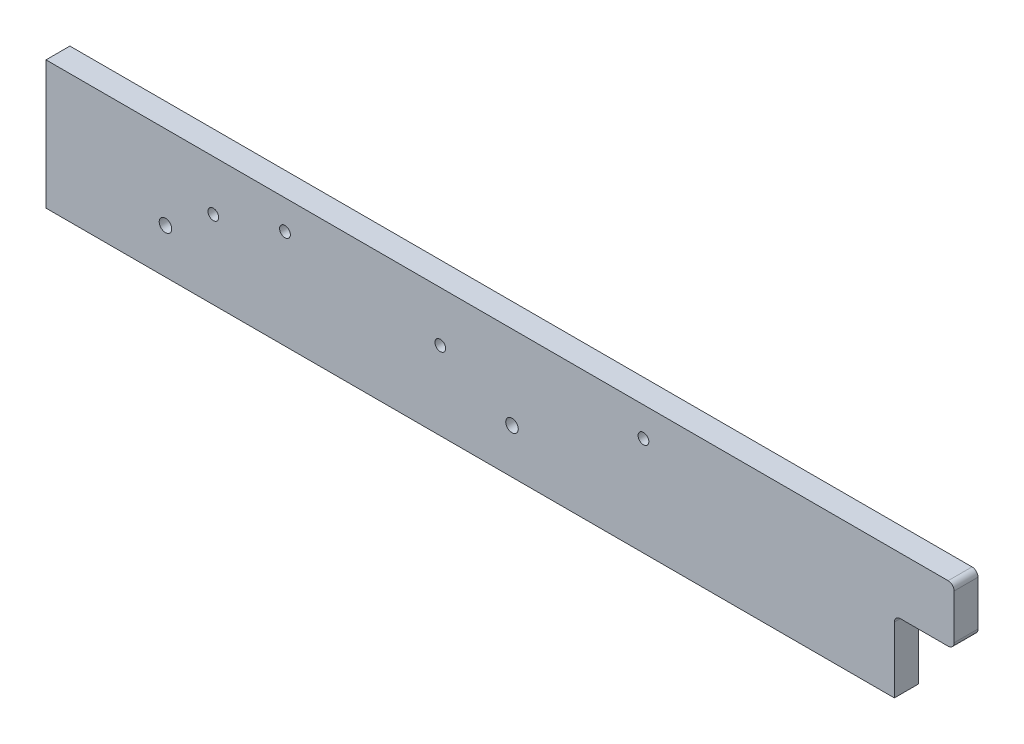
SolidWorks part; units mm, degrees
material "Q235B"
ref_plane "Front Plane" through (0, 0, 0) normal (0, 0, 1) x (1, 0, 0)
ref_plane "Top Plane" through (0, 0, 0) normal (0, 1, 0) x (1, 0, 0)
ref_plane "Right Plane" through (0, 0, 0) normal (1, 0, 0) x (0, 0, -1)
sketch "Sketch1" plane through (0, 0, 0) normal (0, 0, 1) x (1, 0, 0)
  line L0 (0, 215) -> (1520, 215)
  line L1 (0, 0) -> (1420, 0)
  line L2 (0, 0) -> (0, 215)
  line L3 (1420, 0) -> (1420, 120)
  line L5 (1420, 120) -> (1520, 120)
  line L6 (1520, 120) -> (1520, 215)
  circle A0 centre (400, 166) radius 9
  circle A1 centre (280, 131) radius 9
  circle A2 centre (660, 131) radius 9
  circle A3 centre (1000, 166) radius 9
  dimension "D3" = 100
  dimension "D4" = 120
  dimension "D5" = 35
  dimension "D6" = 18
  dimension "D7" = 18
  dimension "D8" = 380
  dimension "D9" = 280
  dimension "D10" = 131
  dimension "D11" = 131
  dimension "D12" = 18
  dimension "D13" = 35
  dimension "D14" = 18
  dimension "D15" = 400
  dimension "D16" = 600
  dimension "D1" = 1420
  dimension "D2" = 215
extrude "Boss-Extrude1" add sketch "Sketch1" along normal blind 40
hole_wizard "M24 Tapped Hole1" positions "3DSketch1" profile "Sketch2" tap size "M24" standard "GB" end condition up to next
sketch3d "3DSketch1"
  point P14 (780, 75, 40)
  point P16 (200, 75, 40)
sketch "Sketch2" plane through (780, 75, 40) normal (1, 0, 0) x (0, -1, 0)
  line L0 (0, 0) -> (0, 40)
  line L1 (0, 40) -> (10.5, 40)
  line L2 (10.5, 40) -> (10.5, 0)
  line L5 (10.5, 0) -> (0, 0)
  line L11 (0, -6.35) -> (0, 107.95) construction
  dimension "通孔螺纹孔钻头直径" = 21
  dimension "通孔螺纹孔钻头深度" = 40
cosmetic thread "Hole thread 3" parameters "D2"=24
cosmetic thread "Hole thread 4" parameters "D2"=24
fillet "Fillet1" radius 10 3 edges at (1520, 215, 20) (1520, 120, 20) (1420, 120, 20)
sketch "Sketch3" plane through (0, 0, 0) normal (0, 0, -1) x (-1, 0, 0)
  circle A0 centre (-1000, 166) radius 9
  circle A1 centre (-400, 166) radius 9.681
extrude "Boss-Extrude2" add sketch "Sketch3" against normal blind 25
hole_wizard "M14 Tapped Hole1" positions "3DSketch2" profile "Sketch4" tap size "M14" standard "GB" end condition up to next
sketch3d "3DSketch2"
  line L0 (1000, 166, 40) -> (1000, 166, 25) construction
  line L1 (400, 166, 40) -> (400, 166, 25) construction
  point P0 (1000, 166, 40)
  point P4 (400, 166, 25)
sketch "Sketch4" plane through (1000, 166, 40) normal (1, 0, 0) x (0, -1, 0)
  line L0 (0, 0) -> (0, 40)
  line L1 (0, 40) -> (6, 40)
  line L2 (6, 40) -> (6, 0)
  line L5 (6, 0) -> (0, 0)
  line L11 (0, -6.35) -> (0, 107.95) construction
  dimension "通孔螺纹孔钻头直径" = 12
  dimension "通孔螺纹孔钻头深度" = 40
cosmetic thread "Hole thread 5" parameters "D2"=14
cosmetic thread "Hole thread 6" parameters "D2"=14
